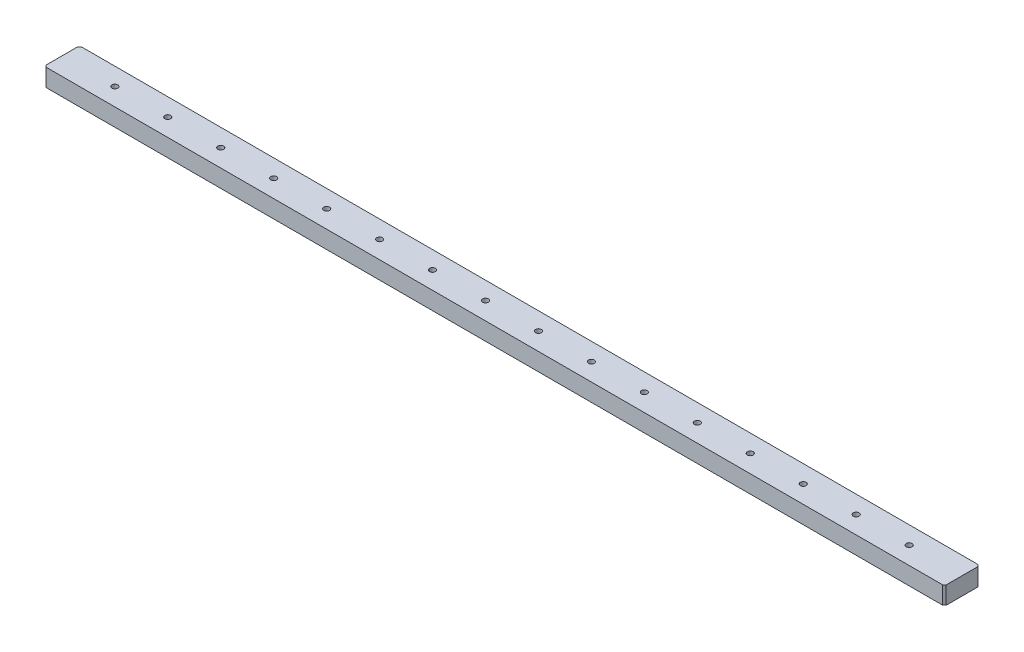
from build123d import *

# Parameters (mm, degrees)
SKETCH_1_W                   = 1020
SKETCH_1_H                   = 40
EXTRUDE_1_DEPTH              = 20
CHAMFER_1_SIZE               = 2
F_4_0MM_1_D                  = 4
F_4_0MM_1_DEPTH              = 12
F_4_0MM_1_TIP                = 1.201721238
PATTERN_LINEAR_5_COUNT       = 17
PATTERN_LINEAR_5_PITCH       = 60
HOLE_WIZARD_M6_1_D           = 6.6
HOLE_WIZARD_M6_1_CBORE_D     = 11
HOLE_WIZARD_M6_1_CBORE_DEPTH = 6.8
PATTERN_LINEAR_6_COUNT       = 16
PATTERN_LINEAR_6_PITCH       = 60


with BuildPart() as part:
    # 草图1 → 凸台-拉伸1 (new body)
    with BuildSketch(Plane(origin=(0, 0, 0), x_dir=(1, 0, 0), z_dir=(0, 1, 0))):
        Rectangle(SKETCH_1_W, SKETCH_1_H)
    extrude(amount=EXTRUDE_1_DEPTH)

    # 倒角1
    chamfer_1_edges = [part.edges().sort_by_distance(p)[0] for p in [
        (510, 10, 20),
        (-510, 10, 20),
        (-510, 10, -20),
        (510, 10, -20),
    ]]
    chamfer(chamfer_1_edges, length=CHAMFER_1_SIZE)

    # Ø4.0mm 暗销孔1
    with Locations(Plane(origin=(0, 0, 0), x_dir=(-1, 0, 0), z_dir=(0, -1, 0))):
        with Locations((480, -9.5), (-480, -9.5)):
            Hole(F_4_0MM_1_D / 2, depth=F_4_0MM_1_DEPTH)
            with Locations((0, 0, -(F_4_0MM_1_DEPTH + F_4_0MM_1_TIP / 2))):  # 118° drill point
                Cone(0, F_4_0MM_1_D / 2, F_4_0MM_1_TIP, mode=Mode.SUBTRACT)

    # 草图9 → M3 螺纹孔1 (revolve, cut)
    with BuildSketch(Plane(origin=(480, 0, 0), x_dir=(0, 0, -1), z_dir=(1, 0, 0))):
        Polygon((0, 0), (0, 8.251075774), (1.25, 7.5), (1.25, 0), align=None)
    hole_wizard_m3_1 = revolve(axis=Axis((480, -6.35, 0), (0, 1, 0)), mode=Mode.SUBTRACT)

    # 阵列(线性)5: M3 螺纹孔1 ×17
    with Locations(*[(-i * PATTERN_LINEAR_5_PITCH, 0, 0) for i in range(1, PATTERN_LINEAR_5_COUNT)]):
        add(hole_wizard_m3_1, mode=Mode.SUBTRACT)

    # M6 六角圆柱头螺钉的柱形沉头孔1 (through all)
    with Locations(Plane(origin=(0, 0, 0), x_dir=(-1, 0, 0), z_dir=(0, -1, 0))):
        with Locations((-450, 0)):
            hole_wizard_m6_1 = CounterBoreHole(HOLE_WIZARD_M6_1_D / 2, HOLE_WIZARD_M6_1_CBORE_D / 2, HOLE_WIZARD_M6_1_CBORE_DEPTH)

    # 阵列(线性)6: M6 六角圆柱头螺钉的柱形沉头孔1 ×16
    with Locations(*[(-i * PATTERN_LINEAR_6_PITCH, 0, 0) for i in range(1, PATTERN_LINEAR_6_COUNT)]):
        add(hole_wizard_m6_1, mode=Mode.SUBTRACT)


solid = part.part
